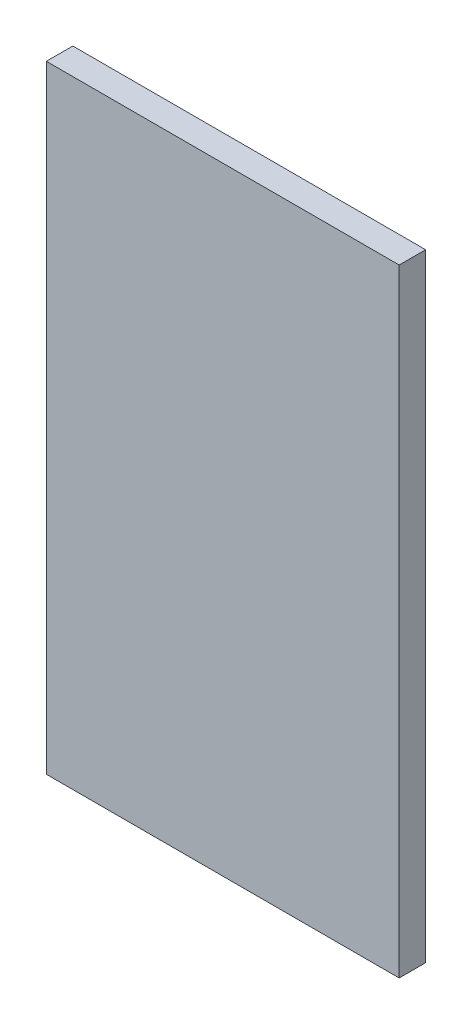
from build123d import *

# Parameters (mm, degrees)
SKETCH_1_W      = 40
SKETCH_1_H      = 70
EXTRUDE_1_DEPTH = 3


with BuildPart() as part:
    # 草图1 → 凸台-拉伸1 (new body)
    with BuildSketch(Plane.XY):
        with Locations((20, 35)):
            Rectangle(SKETCH_1_W, SKETCH_1_H)
    extrude(amount=EXTRUDE_1_DEPTH)


solid = part.part
